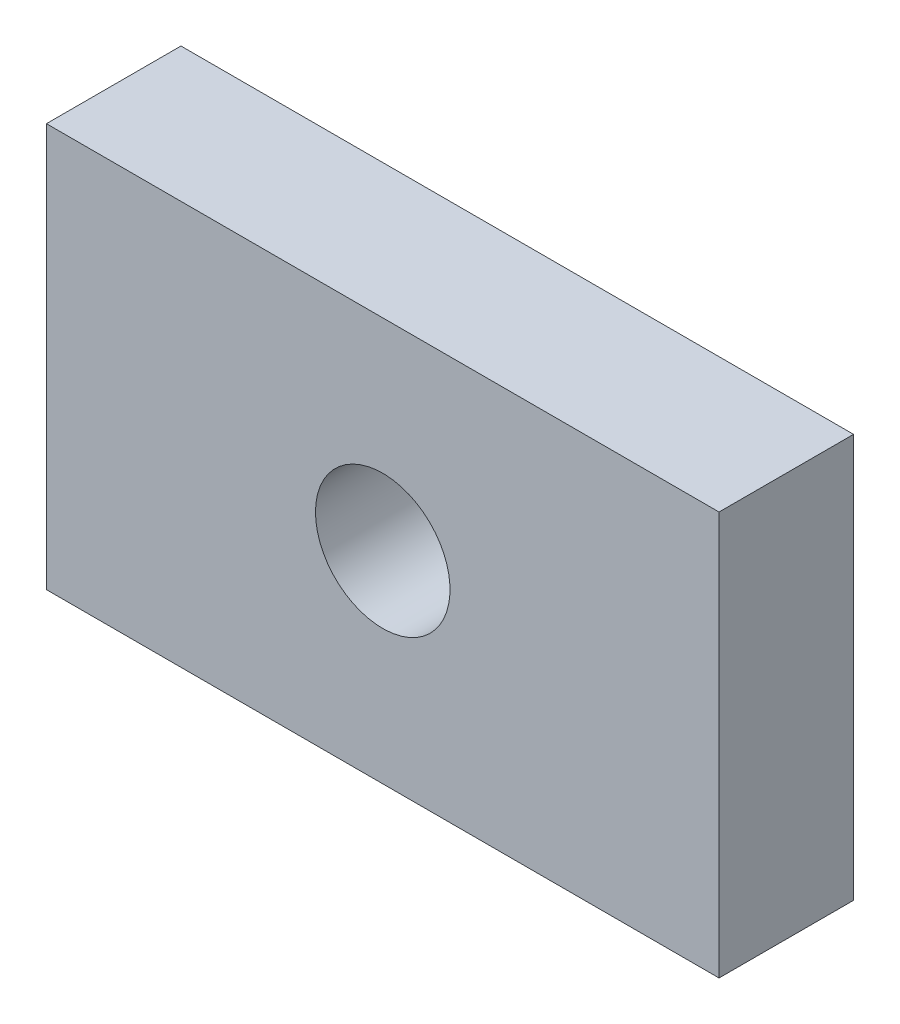
from build123d import *

# Parameters (mm, degrees)
SKETCH1_W           = 50
SKETCH1_H           = 30
SKETCH1_R           = 5
BOSS_EXTRUDE1_DEPTH = 10


with BuildPart() as part:
    # Sketch1 → Boss-Extrude1 (new body)
    with BuildSketch(Plane.XY.offset(5)):
        Rectangle(SKETCH1_W, SKETCH1_H)
        with Locations(Location((0, 0, 0), (0, 0, 180))):
            Circle(SKETCH1_R, mode=Mode.SUBTRACT)
    extrude(amount=-BOSS_EXTRUDE1_DEPTH)


solid = part.part
